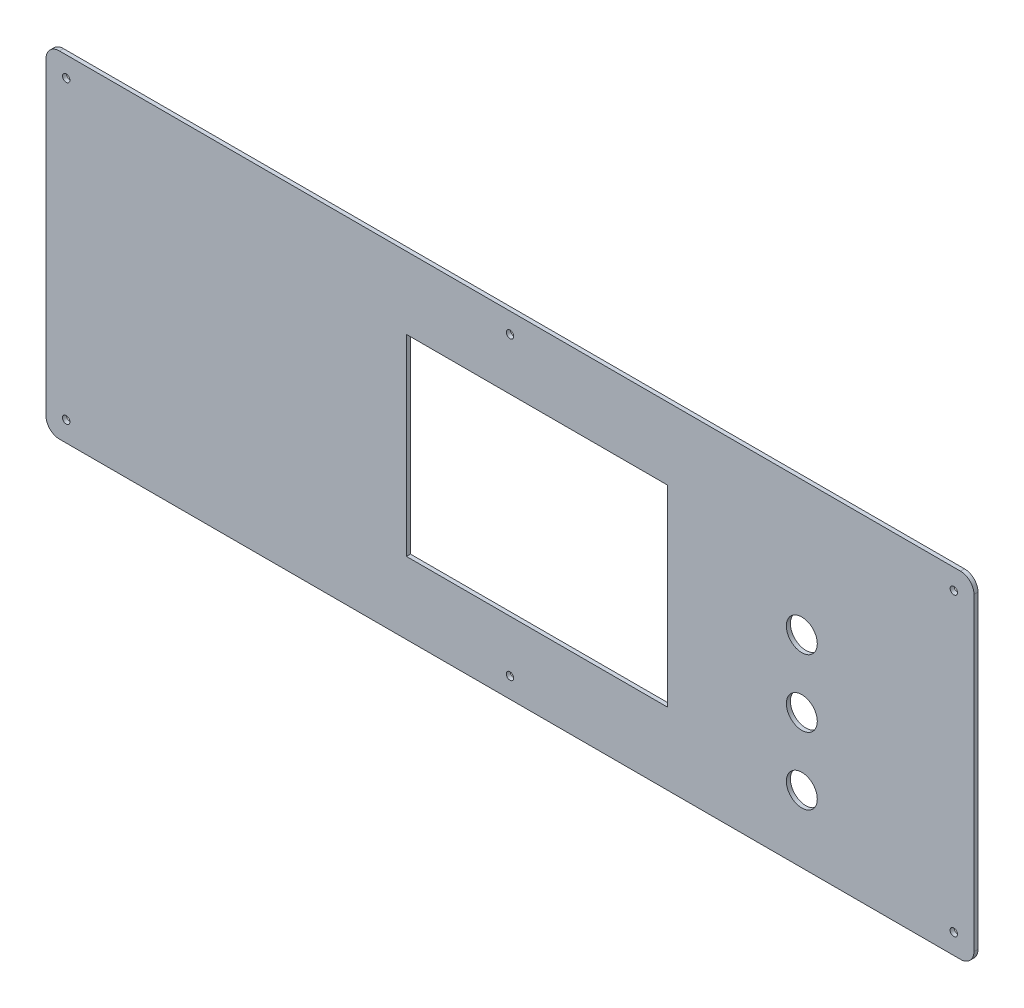
SolidWorks part; units mm, degrees
material "SPCC"
ref_plane "前基準面" through (0, 0, 0) normal (0, 0, 1) x (1, 0, 0)
ref_plane "上基準面" through (0, 0, 0) normal (0, 1, 0) x (1, 0, 0)
ref_plane "右基準面" through (0, 0, 0) normal (1, 0, 0) x (0, 0, -1)
sketch "草图1" plane through (0, 0, 0) normal (0, 0, 1) x (1, 0, 0)
  line L1 (-345, 125) -> (345, 125)
  line L2 (-345, 125) -> (-345, -125)
  line L3 (-345, -125) -> (345, -125)
  line L4 (345, 125) -> (345, -125)
  line L5 (-345, 125) -> (345, -125) construction
  line L6 (-345, -125) -> (345, 125) construction
  point P0 (0, 0)
  dimension "D1" = 690
  dimension "D2" = 250
extrude "凸台-拉伸1" add sketch "草图1" along normal mid plane 3
sketch "草图2" plane through (0, 0, 1.5) normal (0, 0, 1) x (1, 0, 0)
  line L0 (345, -125) -> (345, 125) construction
  line L1 (-77, 71.5) -> (117, 71.5)
  line L2 (-77, 71.5) -> (-77, -71.5)
  line L3 (-77, -71.5) -> (117, -71.5)
  line L4 (117, 71.5) -> (117, -71.5)
  line L5 (-77, 71.5) -> (117, -71.5) construction
  line L6 (-77, -71.5) -> (117, 71.5) construction
  point P0 (20, 0)
  dimension "D1" = 228
  dimension "D2" = 194
  dimension "D3" = 143
extrude "切除-拉伸1" cut sketch "草图2" against normal blind 6
sketch "草图3" plane through (0, 0, 1.5) normal (0, 0, 1) x (1, 0, 0)
  line L0 (117, -71.5) -> (117, 71.5) construction
  line L1 (217, 235.9685) -> (217, -240.6996) construction
  line L3 (-345, -125) -> (345, -125) construction
  circle A0 centre (217, 75) radius 11.5 construction
  arc A1 (205.9929, 28.3308) -> (225.7502, 32.4622) centre (217, 25) ccw
  circle A2 centre (217, -25) radius 11.5
  circle A3 centre (217, -75) radius 11.5
  arc A4 (225.7502, 32.4622) -> (205.9929, 28.3308) centre (217, 25) ccw
  dimension "D6" = 23
  dimension "D7" = 23
  dimension "D2" = 50
  dimension "D3" = 50
  dimension "D4" = 50
  dimension "D5" = 100
  dimension "D11" = 50
extrude "切除-拉伸2" cut sketch "草图3" against normal blind 6
fillet "圆角1" radius 10 4 edges at (345, -125, 0) (345, 125, 0) (-345, -125, 0) (-345, 125, 0)
hole_wizard "Ø5.5 (5.5) 直径孔1" positions "草图6" profile "草图5" hole size "Ø5.5" standard "GB"
sketch "草图6" plane through (0, 0, 1.5) normal (0, 0, 1) x (1, 0, 0)
  line L0 (0, 0) -> (-422.5107, 0) construction
  line L1 (0, 0) -> (0, 177.9278) construction
  line L2 (335, 125) -> (-335, 125) construction
  point P0 (-330, 110)
  point P1 (0, 110)
  point P13 (330, 110)
  point P18 (330, -110)
  point P19 (0, -110)
  point P20 (-330, -110)
  dimension "D1" = 660
  dimension "D2" = 15
  dimension "D3" = 15
sketch "草图5" plane through (-330, 110, 1.5) normal (1, 0, 0) x (0, -1, 0)
  line L0 (0, 0) -> (0, 11.6524)
  line L1 (0, 11.6524) -> (2.75, 10)
  line L2 (2.75, 10) -> (2.75, 0)
  line L5 (2.75, 0) -> (0, 0)
  line L10 (0, 11.6524) -> (-2.75, 10) construction
  line L11 (0, -6.35) -> (0, 107.95) construction
  dimension "孔直径" = 5.5
  dimension "孔深度" = 10
  dimension "导头角度" = 118
